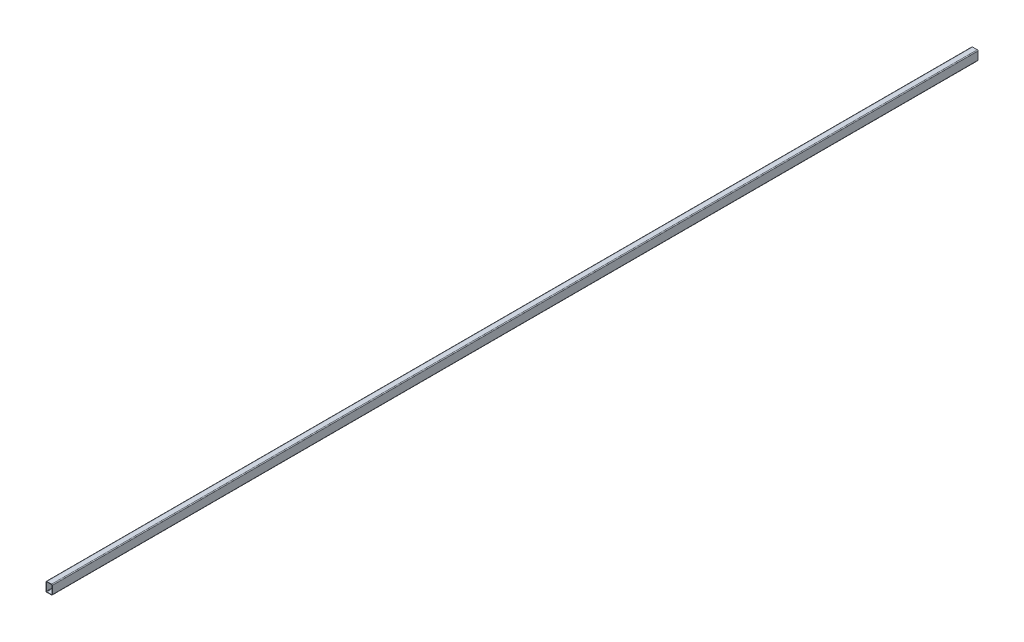
from build123d import *

# Parameters (mm, degrees)
BOSS_EXTRUDE1_DEPTH = 5880


with BuildPart() as part:
    # Sketch1 → Boss-Extrude1 (new body)
    with BuildSketch(Plane.XY):
        with BuildLine():
            Line((5, 0), (35, 0))
            ThreePointArc((35, 0), (38.535533906, 1.464466094), (40, 5))
            Line((40, 5), (40, 55))
            ThreePointArc((40, 55), (38.535533906, 58.535533906), (35, 60))
            Line((35, 60), (5, 60))
            ThreePointArc((5, 60), (1.464466094, 58.535533906), (0, 55))
            Line((0, 55), (0, 5))
            ThreePointArc((0, 5), (1.464466094, 1.464466094), (5, 0))
        make_face()
        with BuildLine():
            Line((5, 2.5), (35, 2.5))
            ThreePointArc((35, 2.5), (36.767766953, 3.232233047), (37.5, 5))
            Line((37.5, 5), (37.5, 55))
            ThreePointArc((37.5, 55), (36.767766953, 56.767766953), (35, 57.5))
            Line((35, 57.5), (5, 57.5))
            ThreePointArc((5, 57.5), (3.232233047, 56.767766953), (2.5, 55))
            Line((2.5, 55), (2.5, 5))
            ThreePointArc((2.5, 5), (3.232233047, 3.232233047), (5, 2.5))
        make_face(mode=Mode.SUBTRACT)
    extrude(amount=BOSS_EXTRUDE1_DEPTH)


solid = part.part
